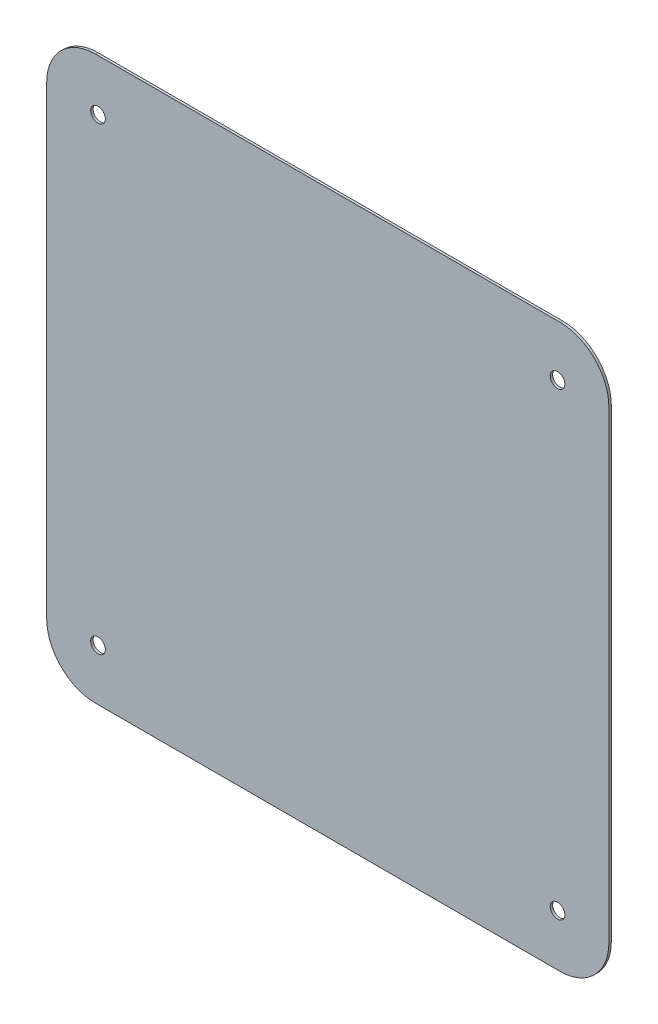
from build123d import *

# Parameters (mm, degrees)
SKETCH1_R           = 1.5
BOSS_EXTRUDE1_DEPTH = 0.5


with BuildPart() as part:
    # Sketch1 → Boss-Extrude1 (new body)
    with BuildSketch(Plane.XY):
        with BuildLine():
            Line((47.5, 57.5), (-47.5, 57.5))
            ThreePointArc((-47.5, 57.5), (-54.571067812, 54.571067812), (-57.5, 47.5))
            Line((-57.5, 47.5), (-57.5, -47.5))
            ThreePointArc((-57.5, -47.5), (-54.571067812, -54.571067812), (-47.5, -57.5))
            Line((-47.5, -57.5), (47.5, -57.5))
            ThreePointArc((47.5, -57.5), (54.571067812, -54.571067812), (57.5, -47.5))
            Line((57.5, -47.5), (57.5, 47.5))
            ThreePointArc((57.5, 47.5), (54.571067812, 54.571067812), (47.5, 57.5))
        make_face()
        with Locations((-47, 47)):
            Circle(SKETCH1_R, mode=Mode.SUBTRACT)
        with Locations((47, 47)):
            Circle(SKETCH1_R, mode=Mode.SUBTRACT)
        with Locations((47, -47)):
            Circle(SKETCH1_R, mode=Mode.SUBTRACT)
        with Locations((-47, -47)):
            Circle(SKETCH1_R, mode=Mode.SUBTRACT)
    extrude(amount=BOSS_EXTRUDE1_DEPTH)


solid = part.part
